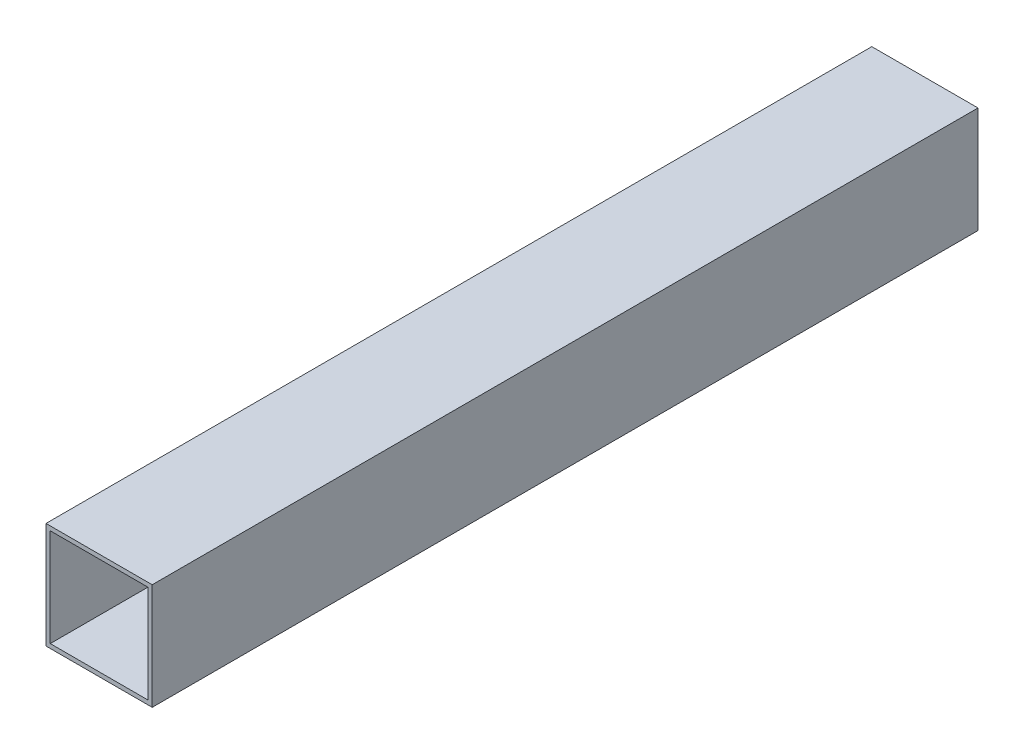
SolidWorks part; units mm, degrees
material "AISI 304"
ref_plane "Front Plane" through (0, 0, 0) normal (0, 0, 1) x (1, 0, 0)
ref_plane "Top Plane" through (0, 0, 0) normal (0, 1, 0) x (1, 0, 0)
ref_plane "Right Plane" through (0, 0, 0) normal (1, 0, 0) x (0, 0, -1)
sketch "Sketch1" plane through (0, 0, 0) normal (0, 0, 1) x (1, 0, 0)
  line L1 (-25, -25) -> (25, -25)
  line L2 (-25, -25) -> (-25, 25)
  line L3 (-25, 25) -> (25, 25)
  line L4 (25, -25) -> (25, 25)
  line L5 (-25, -25) -> (25, 25) construction
  line L6 (-25, 25) -> (25, -25) construction
  line L7 (-23, -23) -> (23, -23)
  line L8 (-23, -23) -> (-23, 23)
  line L9 (-23, 23) -> (23, 23)
  line L10 (23, -23) -> (23, 23)
  line L11 (-23, -23) -> (23, 23) construction
  line L12 (-23, 23) -> (23, -23) construction
  point P0 (0, 0)
  point P6 (0, 0)
  dimension "D1" = 50
  dimension "D2" = 50
  dimension "D3" = 46
  dimension "D4" = 46
extrude "Boss-Extrude1" add sketch "Sketch1" along normal blind 388.8
